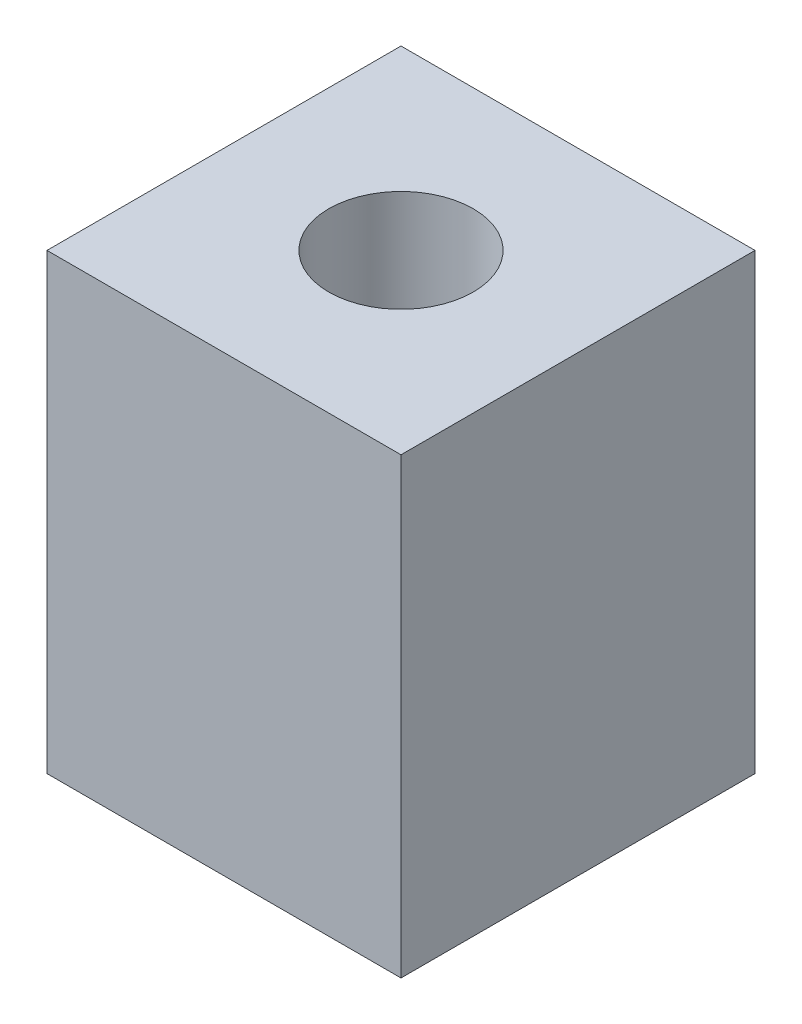
from build123d import *

# Parameters (mm, degrees)
SKETCH1_W           = 25
SKETCH1_H           = 25
BOSS_EXTRUDE1_DEPTH = 32
M12_TAPPED_HOLE1_D  = 10.2


with BuildPart() as part:
    # Sketch1 → Boss-Extrude1 (new body)
    with BuildSketch(Plane(origin=(0, 0, 0), x_dir=(1, 0, 0), z_dir=(0, 1, 0))):
        Rectangle(SKETCH1_W, SKETCH1_H)
    extrude(amount=BOSS_EXTRUDE1_DEPTH)

    # M12 Tapped Hole1 (through all)
    with Locations(Plane(origin=(0, 32, 0), x_dir=(1, 0, 0), z_dir=(0, 1, 0))):
        with Locations((0, 0)):
            Hole(M12_TAPPED_HOLE1_D / 2)


solid = part.part
